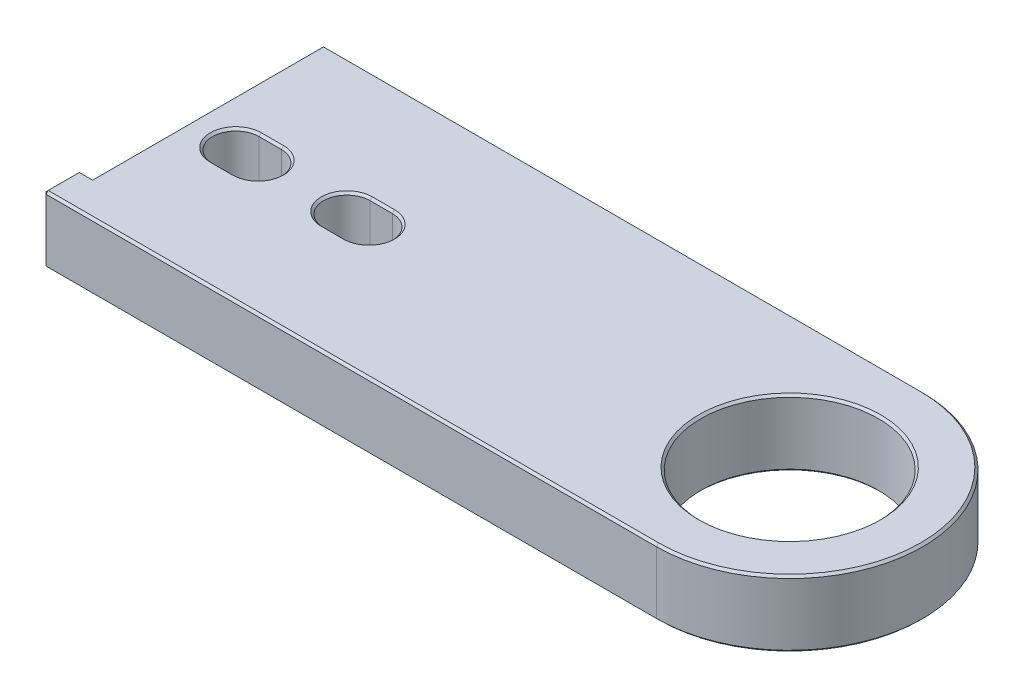
SolidWorks part; units mm, degrees
material "合金钢"
ref_plane "前视基准面" through (0, 0, 0) normal (0, 0, 1) x (1, 0, 0)
ref_plane "上视基准面" through (0, 0, 0) normal (0, 1, 0) x (1, 0, 0)
ref_plane "右视基准面" through (0, 0, 0) normal (1, 0, 0) x (0, 0, -1)
sketch "草图1" plane through (0, 0, 0) normal (0, 1, 0) x (1, 0, 0)
  line L0 (-135, 30) -> (-135, -30)
  line L1 (-135, 30) -> (0, 30)
  line L2 (-135, -30) -> (0, -30)
  line L3 (-124.75, 5.25) -> (-119.75, 5.25)
  line L4 (-124.75, -5.25) -> (-119.75, -5.25)
  line L5 (-99.75, 5.25) -> (-94.75, 5.25)
  line L6 (-99.75, -5.25) -> (-94.75, -5.25)
  circle A0 centre (0, 0) radius 20
  arc A1 (0, -30) -> (0, 30) centre (0, 0) ccw
  arc A2 (-119.75, -5.25) -> (-119.75, 5.25) centre (-119.75, 0) ccw
  arc A3 (-99.75, 5.25) -> (-99.75, -5.25) centre (-99.75, 0) ccw
  arc A4 (-94.75, -5.25) -> (-94.75, 5.25) centre (-94.75, 0) ccw
  arc A5 (-124.75, 5.25) -> (-124.75, -5.25) centre (-124.75, 0) ccw
  point P7 (-135, 0)
  dimension "D1" = 40
  dimension "D2" = 60
  dimension "D5" = 10.5
  dimension "D7" = 10.5
  dimension "D8" = 20
  dimension "D3" = 60
  dimension "D4" = 135
  dimension "D6" = 10.25
  dimension "D9" = 5
  dimension "D10" = 5
extrude "凸台-拉伸1" add sketch "草图1" along normal blind 15
sketch "草图3" plane through (0, 0, 0) normal (0, -1, 0) x (1, 0, 0)
  line L1 (-135, 30) -> (-138, 30)
  line L2 (-135, 30) -> (-135, 22)
  line L3 (-135, 22) -> (-138, 22)
  line L4 (-138, 30) -> (-138, 22)
  dimension "D1" = 8
  dimension "D2" = 3
extrude "凸台-拉伸3" add sketch "草图3" against normal through all
chamfer "倒角2" distance 0.5 angle 45 33 edges at (0, 15, 20) (0, 0, 20) (-122.25, 15, -5.25) (-114.5, 15, 0) (-122.25, 15, 5.25) (-130, 15, 0) (-122.25, 0, -5.25) (-114.5, 0, 0) (-122.25, 0, 5.25) (-130, 0, 0) (-97.25, 15, -5.25) (-89.5, 15, 0) (-97.25, 15, 5.25) (-105, 15, 0) (-97.25, 0, -5.25) (-89.5, 0, 0) (-97.25, 0, 5.25) (-105, 0, 0) (-135, 7.5, -30) (-135, 15, -4) (-67.5, 15, -30) (30, 15, 0) (-69, 15, 30) (-135, 0, -4) (-67.5, 0, -30) (30, 0, 0) (-69, 0, 30) (-138, 7.5, 22) (-136.5, 0, 22) (-136.5, 15, 22) (-138, 0, 26) (-138, 15, 26) (-138, 7.5, 30)
